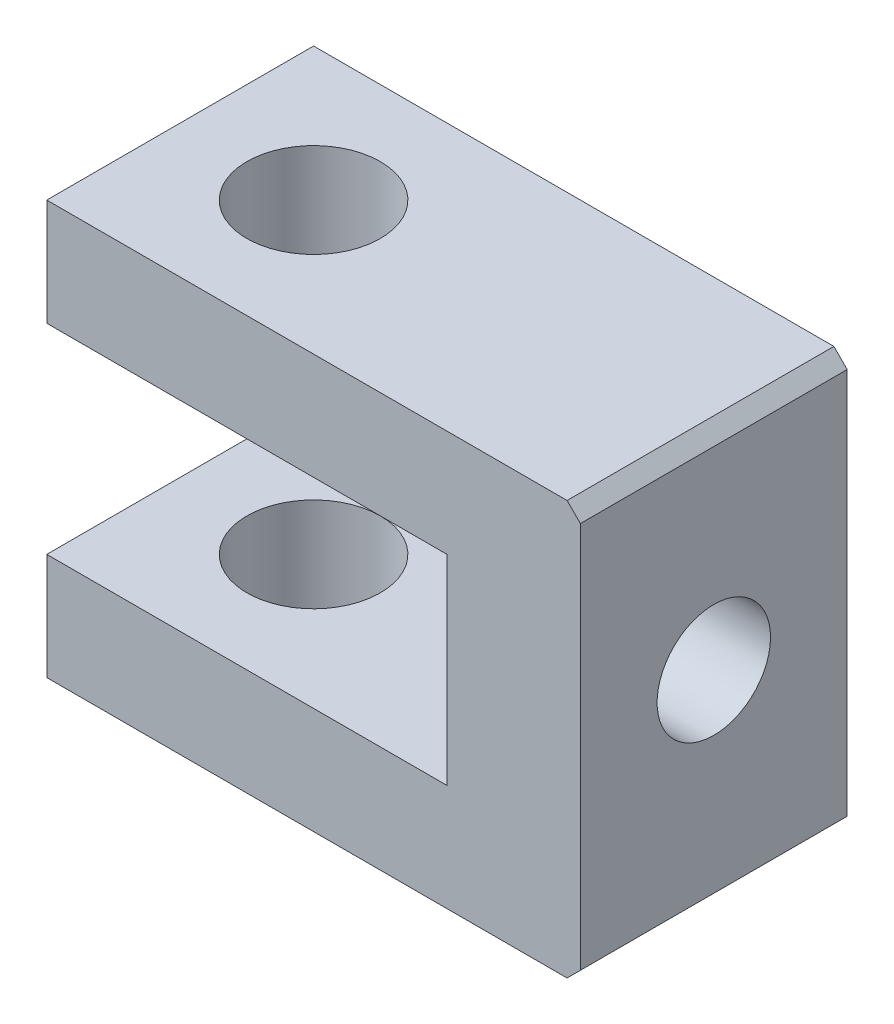
from build123d import *

# Parameters (mm, degrees)
SKETCH_1_W                  = 40
SKETCH_1_H                  = 31
EXTRUDE_1_DEPTH             = 20
SKETCH_2_W                  = 30
SKETCH_2_H                  = 15
CUT_EXTRUDE_1_DEPTH         = 35.220141674
HOLE_WIZARD_10_0_10_1_D     = 10
HOLE_WIZARD_10_0_10_1_DEPTH = 8
HOLE_WIZARD_8_5_8_5_1_D     = 8.5
HOLE_WIZARD_8_5_8_5_1_DEPTH = 40
HOLE_WIZARD_10_0_10_2_D     = 10
CHAMFER_1_SIZE              = 1


with BuildPart() as part:
    # 草图1 → 凸台-拉伸1 (new body)
    with BuildSketch(Plane(origin=(0, 0, -10), x_dir=(-1, 0, 0), z_dir=(0, 0, -1))):
        with Locations((-3.03840481, 0)):
            Rectangle(SKETCH_1_W, SKETCH_1_H)
    extrude(amount=-EXTRUDE_1_DEPTH)

    # 草图2 → 切除-拉伸1 (cut, through all)
    with BuildSketch(Plane.XY.offset(10)):
        with Locations((-1.96159519, 0)):
            Rectangle(SKETCH_2_W, SKETCH_2_H)
    extrude(amount=-CUT_EXTRUDE_1_DEPTH, mode=Mode.SUBTRACT)

    # Ø10.0 (10) 直径孔1
    with Locations(Plane(origin=(0, -15.5, 0), x_dir=(-1, 0, 0), z_dir=(0, -1, 0))):
        with Locations((6.96159519, 0)):
            Hole(HOLE_WIZARD_10_0_10_1_D / 2, depth=HOLE_WIZARD_10_0_10_1_DEPTH)

    # Ø8.5 (8.5) 直径孔1
    with Locations(Plane(origin=(23.03840481, 0, 0), x_dir=(0, 0, -1), z_dir=(1, 0, 0))):
        with Locations((0, 0)):
            Hole(HOLE_WIZARD_8_5_8_5_1_D / 2, depth=HOLE_WIZARD_8_5_8_5_1_DEPTH)

    # Ø10.0 (10) 直径孔2 (through all)
    with Locations(Plane(origin=(0, 7.5, 0), x_dir=(-1, 0, 0), z_dir=(0, -1, 0))):
        with Locations((6.96159519, 0)):
            Hole(HOLE_WIZARD_10_0_10_2_D / 2)

    # 倒角1
    chamfer_1_edges = [part.edges().sort_by_distance(p)[0] for p in [
        (23.03840481, -15.5, 0),
        (23.03840481, 15.5, 0),
    ]]
    chamfer(chamfer_1_edges, length=CHAMFER_1_SIZE)


solid = part.part
